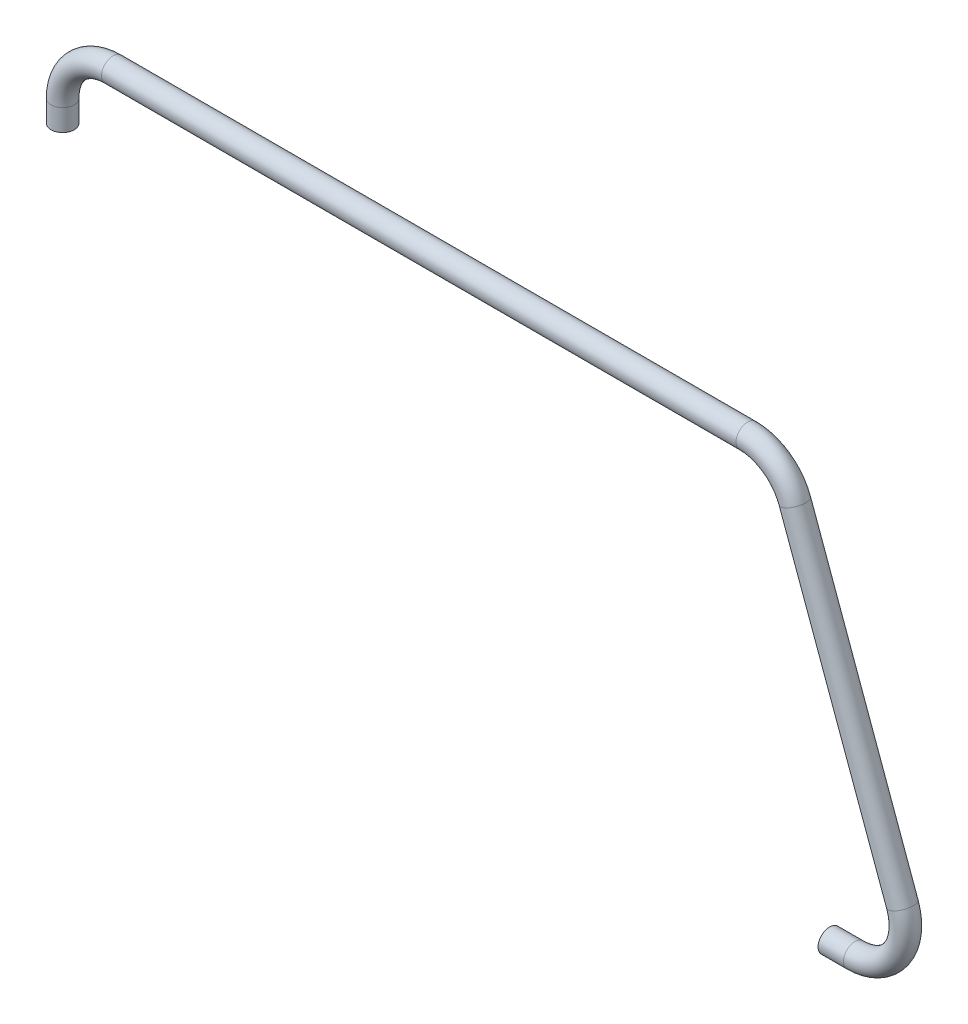
from build123d import *

# Parameters (mm, degrees)
SKETCH2_R   = 16
SKETCH2_R_2 = 13


with BuildPart() as part:
    # Sweep1: sweep along a path in Sketch1
    with BuildLine(Plane.XY) as sweep1_path:
        Line((0, 0), (0, 30))
        ThreePointArc((0, 30), (20.502525317, 79.497474683), (70, 100))
        Line((70, 100), (950.985472325, 100))
        ThreePointArc((950.985472325, 100), (991.13582287, 87.3406431), (1016.76395578, 53.941410033))
        Line((1016.76395578, 53.941410033), (1165.991751829, -356.058589967))
        ThreePointArc((1165.991751829, -356.058589967), (1157.553911475, -420.150350545), (1100.213268374, -450))
        Line((1100.213268374, -450), (1065, -450))
    # Sketch2 → Sweep1 (sweep)
    with BuildSketch(Plane(origin=(0, 0, 0), x_dir=(1, 0, 0), z_dir=(0, 1, 0))):
        Circle(SKETCH2_R)
        Circle(SKETCH2_R_2, mode=Mode.SUBTRACT)
    sweep(path=sweep1_path.line)


solid = part.part
